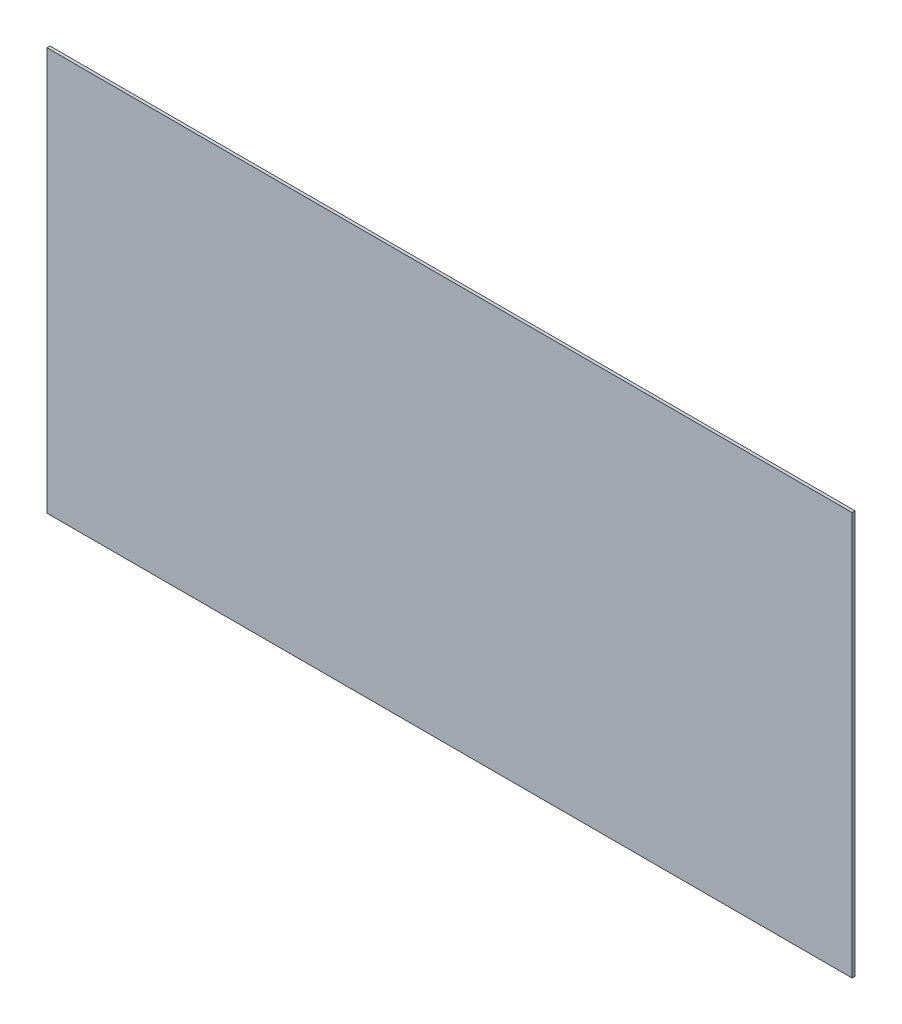
from build123d import *

# Parameters (mm, degrees)
SKETCH_1_W      = 1350
SKETCH_1_H      = 676
EXTRUDE_1_DEPTH = 5


with BuildPart() as part:
    # 草图1 → 凸台-拉伸1 (new body)
    with BuildSketch(Plane.XY):
        Rectangle(SKETCH_1_W, SKETCH_1_H)
    extrude(amount=EXTRUDE_1_DEPTH)


solid = part.part
